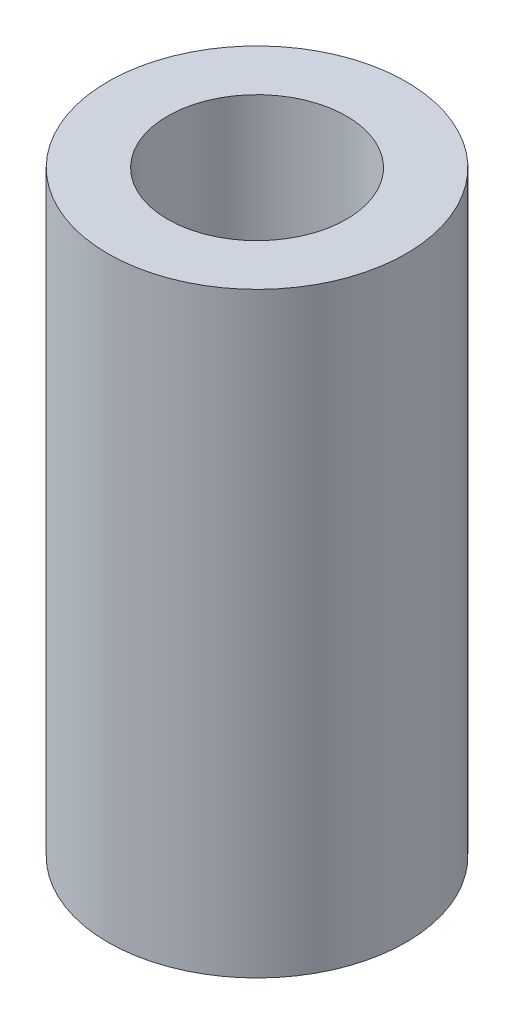
SolidWorks part; units mm, degrees
material "ABS"
ref_plane "前视基准面" through (0, 0, 0) normal (0, 0, 1) x (1, 0, 0)
ref_plane "上视基准面" through (0, 0, 0) normal (0, 1, 0) x (1, 0, 0)
ref_plane "右视基准面" through (0, 0, 0) normal (1, 0, 0) x (0, 0, -1)
sketch "草图1" plane through (0, 0, 0) normal (0, 1, 0) x (1, 0, 0)
  circle A0 centre (0, 0) radius 1.5
  circle A1 centre (0, 0) radius 2.5
  dimension "D1" = 3
  dimension "D2" = 5
extrude "凸台-拉伸1" add sketch "草图1" along normal blind 10
